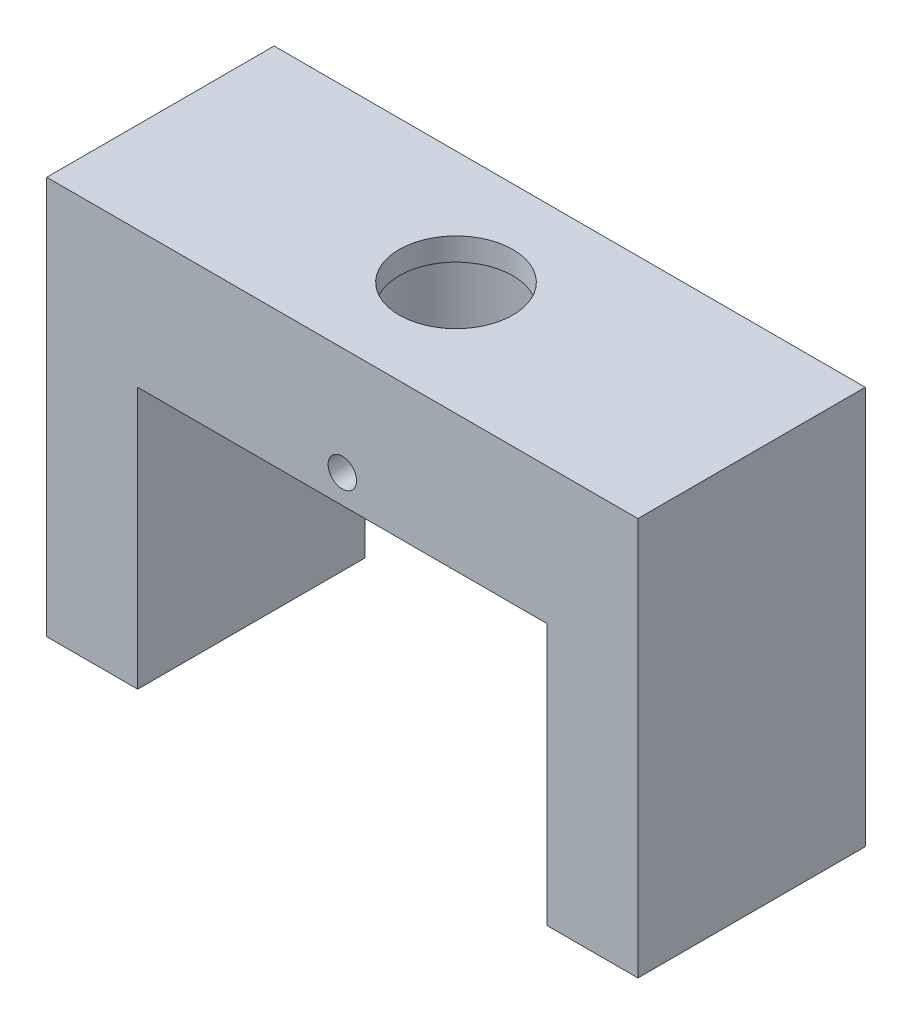
from build123d import *

# Parameters (mm, degrees)
BOSS_EXTRUDE1_DEPTH    = 10
SKETCH3_R              = 5
CUT_EXTRUDE2_DEPTH     = 27
SKETCH5_R              = 1.5
CUT_EXTRUDE4_DEPTH     = 10
M4_TAPPED_HOLE1_D      = 3.3
M4_TAPPED_HOLE1_DEPTH  = 10
M4_TAPPED_HOLE1_TIP    = 0.991420021
SKETCH9_R              = 7.5
CUT_EXTRUDE5_DEPTH     = 10
M3_TAPPED_HOLE2_REACH  = 45.296
M3_TAPPED_HOLE2_BORE_R = 1.25
M3_TAPPED_HOLE3_D      = 2.5
M3_TAPPED_HOLE3_DEPTH  = 10
M3_TAPPED_HOLE3_TIP    = 0.751075774


with BuildPart() as part:
    # Sketch1 → Boss-Extrude1 (new, symmetric)
    with BuildSketch(Plane.XY):
        Polygon((-18, -6.74079026), (-26, -6.74079026), (-26, 28.25920974), (26, 28.25920974), (26, -6.74079026), (18, -6.74079026), (18, 16.25920974), (-18, 16.25920974), align=None)
    extrude(amount=BOSS_EXTRUDE1_DEPTH, both=True)

    # Sketch3 → Cut-Extrude2 (cut)
    with BuildSketch(Plane(origin=(0, 28.25920974, 0), x_dir=(1, 0, 0), z_dir=(0, 1, 0))):
        with Locations(Location((0, 0, 0), (0, 0, 180))):
            Circle(SKETCH3_R)
    extrude(amount=-CUT_EXTRUDE2_DEPTH, mode=Mode.SUBTRACT)

    # Sketch5 → Cut-Extrude4 (cut)
    with BuildSketch(Plane.XZ.offset(6.74079026)):
        with Locations((22, 6)):
            Circle(SKETCH5_R)
        with Locations((22, -6)):
            Circle(SKETCH5_R)
        with Locations(Location((-22, -6, 0), (0, 0, 180))):
            Circle(SKETCH5_R)
        with Locations(Location((-22, 6, 0), (0, 0, 180))):
            Circle(SKETCH5_R)
    extrude(amount=-CUT_EXTRUDE4_DEPTH, mode=Mode.SUBTRACT)

    # M4 Tapped Hole1
    with Locations(Plane(origin=(0, -6.74079026, 0), x_dir=(-1, 0, 0), z_dir=(0, -1, 0))):
        with Locations((-22, 6), (-22, -6), (22, 6), (22, -6)):
            Hole(M4_TAPPED_HOLE1_D / 2, depth=M4_TAPPED_HOLE1_DEPTH)
            with Locations((0, 0, -(M4_TAPPED_HOLE1_DEPTH + M4_TAPPED_HOLE1_TIP / 2))):  # 118° drill point
                Cone(0, M4_TAPPED_HOLE1_D / 2, M4_TAPPED_HOLE1_TIP, mode=Mode.SUBTRACT)

    # Sketch9 → Cut-Extrude5 (cut)
    with BuildSketch(Plane.XZ.offset(-16.25920974)):
        Circle(SKETCH9_R)
    extrude(amount=-CUT_EXTRUDE5_DEPTH, mode=Mode.SUBTRACT)

    # M3 Tapped Hole2 bore → M3 Tapped Hole2 (cut, up to next)
    with BuildSketch(Plane.XY.offset(10), mode=Mode.PRIVATE) as m3_tapped_hole2_sk1:
        with Locations((0, 18.75920974)):
            Circle(M3_TAPPED_HOLE2_BORE_R)
    m3_tapped_hole2_tool1 = extrude(m3_tapped_hole2_sk1.sketch, amount=-M3_TAPPED_HOLE2_REACH, mode=Mode.PRIVATE) & part.part
    add(m3_tapped_hole2_tool1.solids().sort_by_distance((0, 18.75921, 10))[0], mode=Mode.SUBTRACT)

    # M3 Tapped Hole3
    with Locations(Plane(origin=(0, 16.25920974, 0), x_dir=(-1, 0, 0), z_dir=(0, -1, 0))):
        with Locations((10, 0), (-10, 0)):
            Hole(M3_TAPPED_HOLE3_D / 2, depth=M3_TAPPED_HOLE3_DEPTH)
            with Locations((0, 0, -(M3_TAPPED_HOLE3_DEPTH + M3_TAPPED_HOLE3_TIP / 2))):  # 118° drill point
                Cone(0, M3_TAPPED_HOLE3_D / 2, M3_TAPPED_HOLE3_TIP, mode=Mode.SUBTRACT)


solid = part.part
